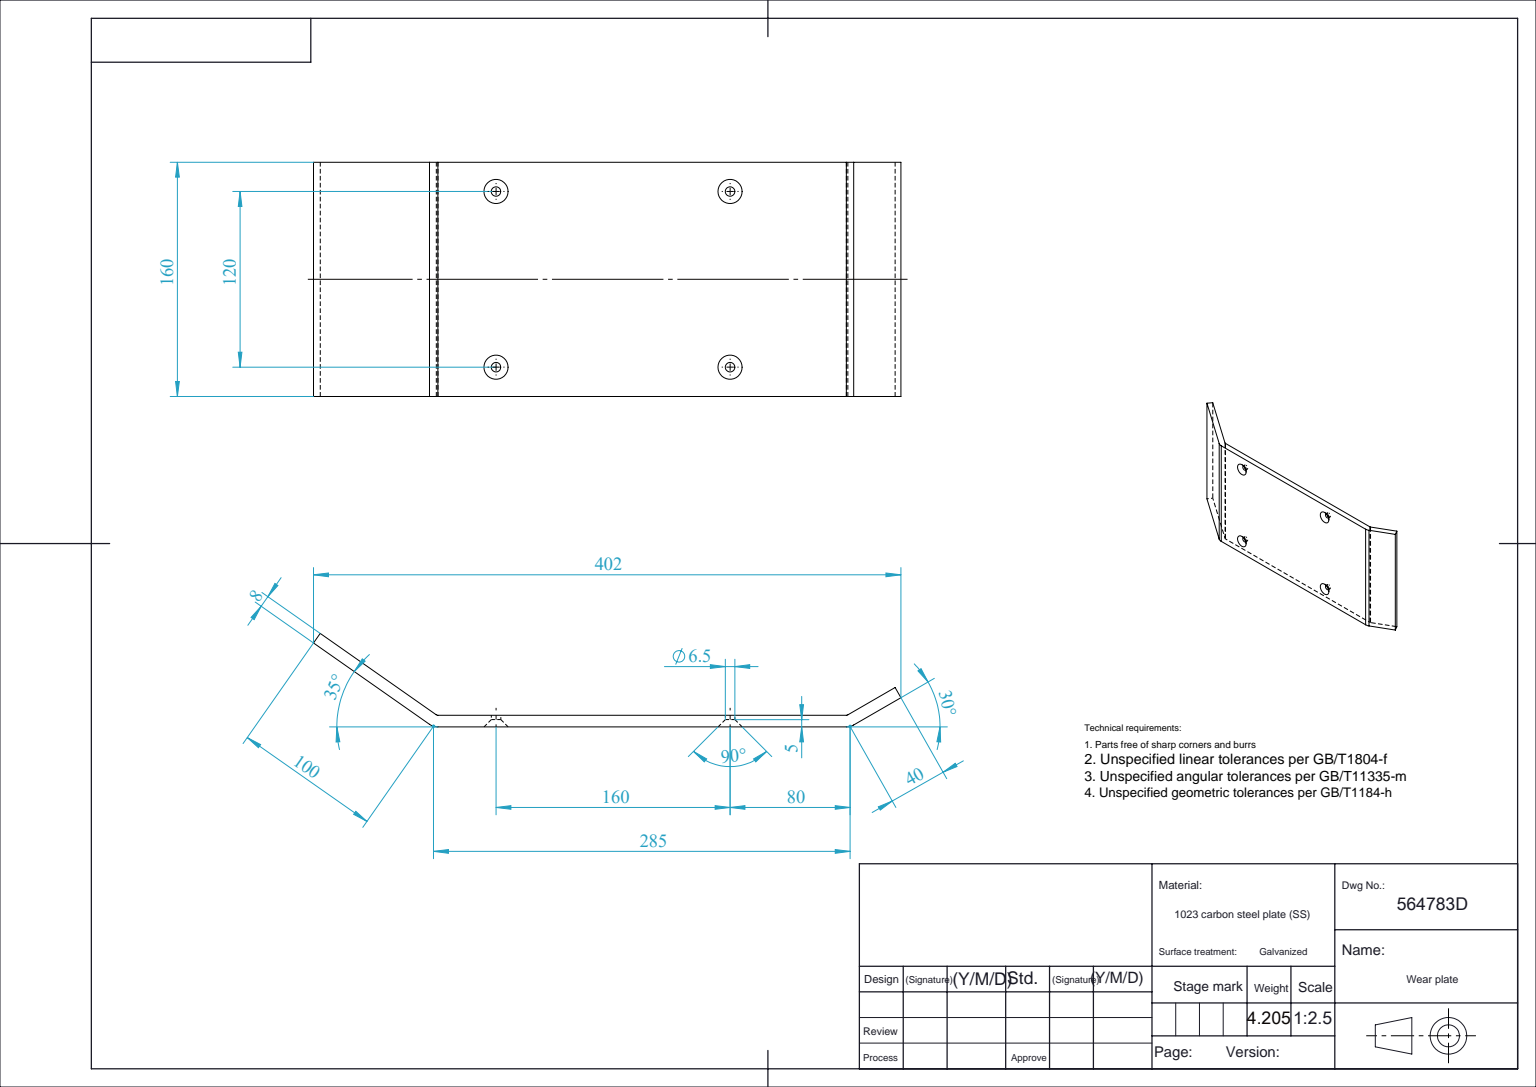
SolidWorks part; units mm, degrees
material "1023 carbon steel plate (SS)"
ref_plane "Front Plane" through (0, 0, 0) normal (0, 0, 1) x (1, 0, 0)
ref_plane "Top Plane" through (0, 0, 0) normal (0, 1, 0) x (1, 0, 0)
ref_plane "Right Plane" through (0, 0, 0) normal (1, 0, 0) x (0, 0, -1)
sketch "Sketch23" plane through (0, 0, 0) normal (0, 0, 1) x (1, 0, 0)
  line L0 (0, 0) -> (81.9152, -57.3576)
  line L1 (81.9152, -57.3576) -> (366.9152, -57.3576)
  line L2 (366.9152, -57.3576) -> (401.5562, -37.3576)
  line L3 (4.5886, 6.5532) -> (84.4376, -49.3576)
  line L4 (84.4376, -49.3576) -> (364.7716, -49.3576)
  line L5 (364.7716, -49.3576) -> (397.5562, -30.4294)
  line L6 (4.5886, 6.5532) -> (-0.4438, -0.6338)
  line L7 (397.5562, -30.4294) -> (401.5562, -37.3576)
  dimension "D1" = 285
  dimension "D2" = 100
  dimension "D3" = 40
  dimension "D4" = 35
  dimension "D5" = 30
  dimension "D7" = 402
  dimension "D6" = 8
extrude "Boss-Extrude4" add sketch "Sketch23" along normal blind 160 contours L7 L5 L4 L3 L6 L0 L1 L2
sketch "Sketch24" plane through (0, -49.3576, 0) normal (0, 1, 0) x (1, 0, 0)
  line L0 (364.7716, -160) -> (364.7716, 0) construction
  line L1 (84.4376, 0) -> (364.7716, 0) construction
  circle A0 centre (124.7716, -20) radius 3.25
  circle A1 centre (284.7716, -20) radius 3.25
  circle A2 centre (124.7716, -140) radius 3.25
  circle A3 centre (284.7716, -140) radius 3.25
  dimension "D1" = 6.5
  dimension "D2" = 160
  dimension "D3" = 80
  dimension "D4" = 120
  dimension "D5" = 20
extrude "Cut-Extrude3" cut sketch "Sketch24" against normal blind 8
sketch "Sketch26" plane through (0, -57.3576, 0) normal (0, -1, 0) x (1, 0, 0)
  circle A0 centre (124.7716, 140) radius 8.25
  circle A1 centre (284.7716, 140) radius 8.25
  circle A2 centre (284.7716, 20) radius 8.25
  circle A3 centre (124.7716, 20) radius 8.25
  dimension "D1" = 16.5
extrude "Cut-Extrude4" cut sketch "Sketch26" against normal blind 5 draft 45
fillet "Fillet1" radius 10 2 edges at (366.9152, -57.3576, 80) (81.9152, -57.3576, 80)
fillet "Fillet2" radius 2 2 edges at (84.4376, -49.3576, 80) (364.7716, -49.3576, 80)
